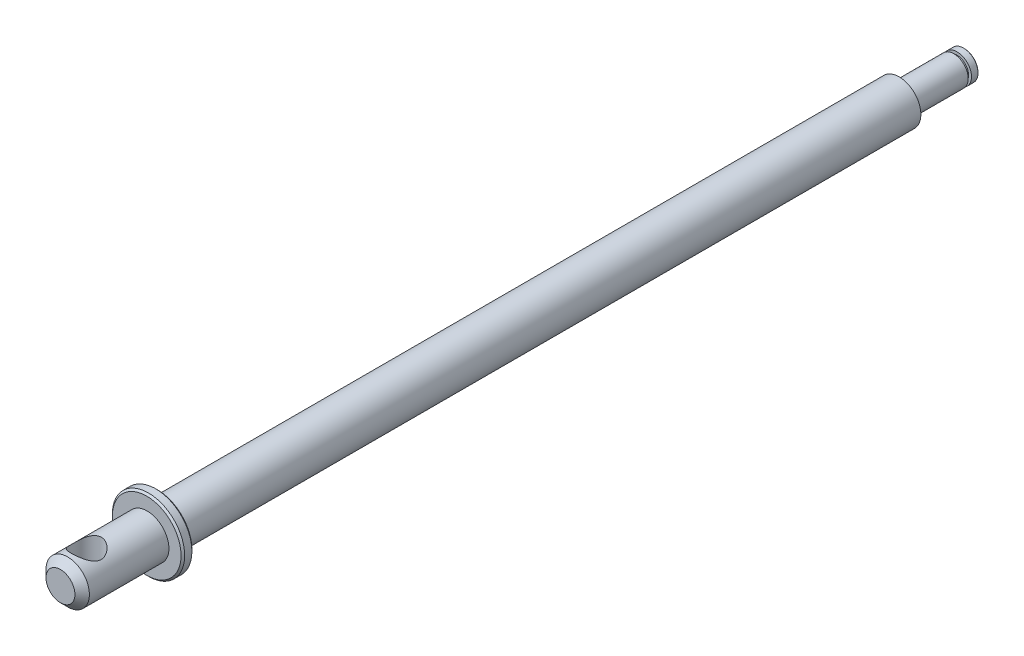
SolidWorks part; units mm, degrees
ref_plane "Plan de face" through (0, 0, 0) normal (0, 0, 1) x (1, 0, 0)
ref_plane "Plan de dessus" through (0, 0, 0) normal (0, 1, 0) x (1, 0, 0)
ref_plane "Plan de droite" through (0, 0, 0) normal (1, 0, 0) x (0, 0, -1)
sketch "Sketch1" plane through (0, 0, 0) normal (0, 1, 0) x (1, 0, 0)
  line L0 (4.1424, -208.2686) -> (3.3424, -208.2686)
  line L1 (0.1424, -206.2686) -> (4.1424, -206.2686)
  line L2 (4.1424, -224.2686) -> (4.1424, -209.1686)
  line L3 (6.1424, -456.2686) -> (0.1424, -456.2686)
  line L4 (0.1424, -206.2686) -> (0.1424, -456.2686)
  line L5 (3.3424, -208.2686) -> (3.3424, -209.1686)
  line L7 (6.1424, -456.2686) -> (6.1424, -224.2686)
  line L8 (3.3424, -209.1686) -> (4.1424, -209.1686)
  line L10 (4.1424, -208.2686) -> (4.1424, -206.2686)
  line L24 (6.1424, -224.2686) -> (4.1424, -224.2686)
  point P7 (4.1424, -206.2686)
  point P25 (10.1424, -206.2686)
  dimension "D1" = 18
  dimension "D2" = 2
  dimension "D3" = 250
revolve "Revolve1" add sketch "Sketch1" angle 360 about L4
sketch "Sketch4" plane through (0, 0, 0) normal (0, 1, 0) x (1, 0, 0)
  circle A0 centre (0, -448.8942) radius 4
  dimension "D1" = 8
extrude "Cut-Extrude2" cut sketch "Sketch4" against normal mid plane 50
chamfer "Chamfer2" distance 2 angle 45 1 edges at (-5.8576, 0, 456.2686)
chamfer "Chamfer3" distance 0.2 angle 45 1 edges at (-3.8576, 0, 206.2686)
ref_plane "Plan2" through (0, 0, 429.2686) normal (0, 0, 1) x (1, 0, 0)
sketch "Sketch5" plane through (0, 0, 429.2686) normal (0, 0, 1) x (1, 0, 0)
  circle A0 centre (0, 0) radius 10
  dimension "D1" = 20
extrude "Boss.-Extru.1" add sketch "Sketch5" along normal blind 3
chamfer "Chamfer4" distance 0.5 angle 45 2 edges at (10, 0, 429.2686) (10, 0, 432.2686)
